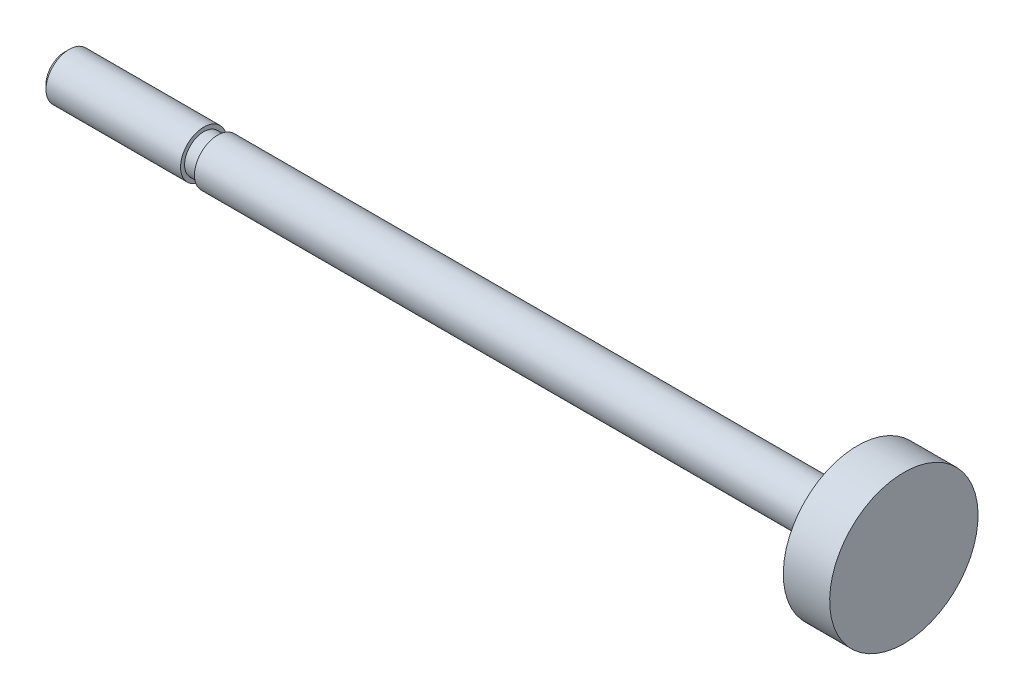
from build123d import *


with BuildPart() as part:
    # Sketch1 → Revolve1 (revolve)
    with BuildSketch(Plane.XY, mode=Mode.PRIVATE) as revolve1_sk:
        Polygon((0, 0), (0, 2.0095), (0.4905, 2.5), (15, 2.5), (15, 2.065), (16.5, 2.065), (16.5, 2.5), (85.5, 2.5), (85.5, 8), (90.5, 8), (90.5, 0), align=None)
    revolve(revolve1_sk.sketch.rotate(Axis((90.5, 0, 0), (-1, 0, 0)), 180), axis=Axis((90.5, 0, 0), (-1, 0, 0)))


solid = part.part
